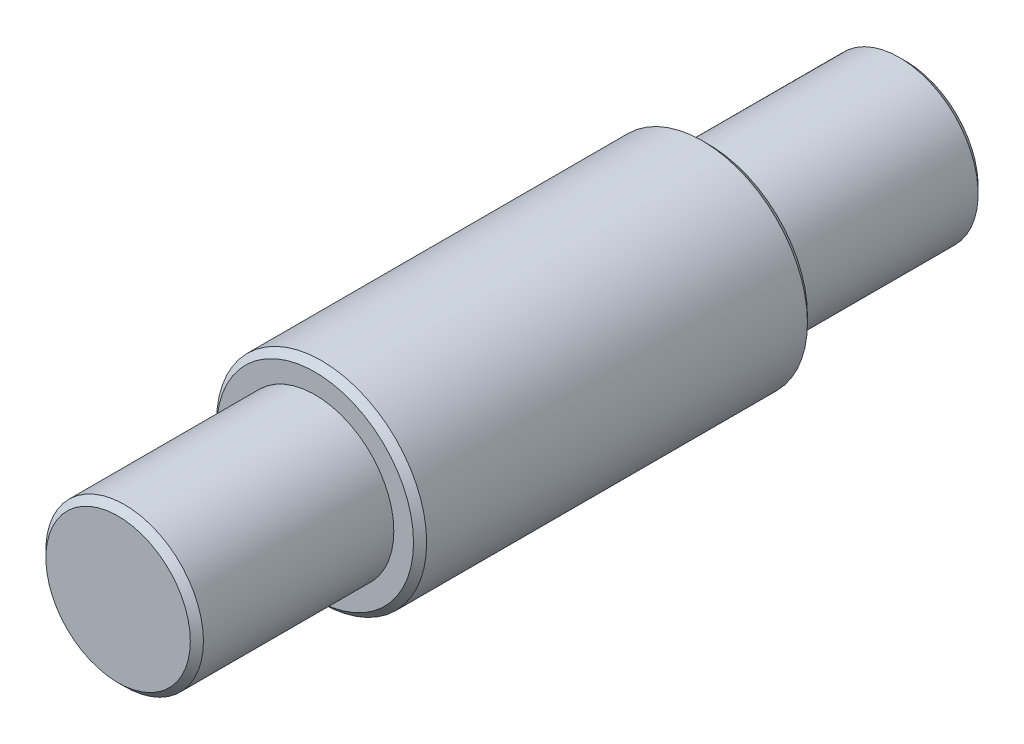
from build123d import *

# Parameters (mm, degrees)
SKETCH1_R           = 6
BOSS_EXTRUDE1_DEPTH = 15
SKETCH2_R           = 8
BOSS_EXTRUDE2_DEPTH = 30
BOSS_EXTRUDE3_START = 15
SKETCH3_R           = 6
BOSS_EXTRUDE3_DEPTH = 15
CHAMFER1_SIZE       = 0.5


with BuildPart() as part:
    # Sketch1 → Boss-Extrude1 (new body)
    with BuildSketch(Plane.XY):
        Circle(SKETCH1_R)
    extrude(amount=BOSS_EXTRUDE1_DEPTH)

    # Sketch2 → Boss-Extrude2 (add)
    with BuildSketch(Plane(origin=(0, 0, 0), x_dir=(-1, 0, 0), z_dir=(0, 0, -1))):
        Circle(SKETCH2_R)
    extrude(amount=BOSS_EXTRUDE2_DEPTH)

    # Sketch3 → Boss-Extrude3 (add)
    with BuildSketch(Plane(origin=(0, 0, -30), x_dir=(-1, 0, 0), z_dir=(0, 0, -1)).offset(BOSS_EXTRUDE3_START)):
        with Locations(Location((0, 0, 0), (0, 0, 180))):
            Circle(SKETCH3_R)
    extrude(amount=-BOSS_EXTRUDE3_DEPTH)

    # Chamfer1
    chamfer1_edges = [part.edges().sort_by_distance(p)[0] for p in [
        (-6, 0, -45),
        (-6, 0, 15),
        (8, 0, 0),
        (8, 0, -30),
    ]]
    chamfer(chamfer1_edges, length=CHAMFER1_SIZE)


solid = part.part
